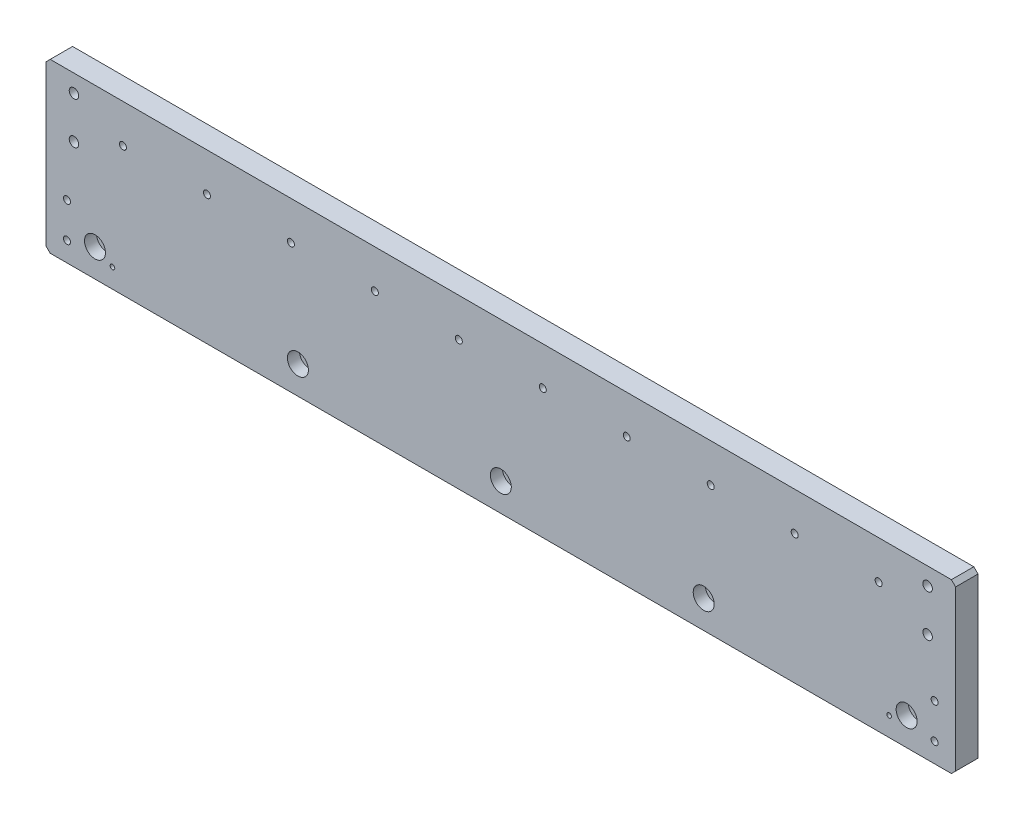
from build123d import *

# Parameters (mm, degrees)
SKETCH_1_W                     = 670
SKETCH_1_H                     = 140
EXTRUDE_1_DEPTH                = 16
HOLE_WIZARD_M8_1_D             = 6.8
HOLE_WIZARD_M6_1_D             = 5
HOLE_WIZARD_M8_1_2_D           = 9
HOLE_WIZARD_M8_1_2_CBORE_D     = 15
HOLE_WIZARD_M8_1_2_CBORE_DEPTH = 8.6
SKETCH_16_W                    = 670
SKETCH_16_H                    = 20
CUT_EXTRUDE_1_DEPTH            = 343.609106709
SKETCH_19_W                    = 10
SKETCH_19_H                    = 120
CUT_EXTRUDE_2_DEPTH            = 343.609106709
CHAMFER_1_SIZE                 = 3
HOLE_WIZARD_M6_2_D             = 5
HOLE_WIZARD_M4_1_D             = 3.3


with BuildPart() as part:
    # 草图1 → 凸台-拉伸1 (new body)
    with BuildSketch(Plane.XY):
        Rectangle(SKETCH_1_W, SKETCH_1_H)
    extrude(amount=EXTRUDE_1_DEPTH)

    # Hole Wizard M8 _1 (through all)
    with Locations(Plane.XY.offset(16)):
        with Locations((-305, 57.5), (-305, 27.5), (305, 27.5), (305, 57.5)):
            Hole(HOLE_WIZARD_M8_1_D / 2)

    # M6 螺纹孔1 (through all)
    with Locations(Plane.XY.offset(16)):
        with Locations((-270, 42.5), (-210, 42.5), (-150, 42.5), (-90, 42.5), (-30, 42.5), (30, 42.5), (90, 42.5), (150, 42.5), (210, 42.5), (270, 42.5)):
            Hole(HOLE_WIZARD_M6_1_D / 2)

    # Hole Wizard M8 _1 2 (through all)
    with Locations(Plane.XY.offset(16)):
        with Locations((290, -30), (145, -30), (0, -30), (-145, -30), (-290, -30), (-435, -30)):
            CounterBoreHole(HOLE_WIZARD_M8_1_2_D / 2, HOLE_WIZARD_M8_1_2_CBORE_D / 2, HOLE_WIZARD_M8_1_2_CBORE_DEPTH)

    # 草图16 → 切除-拉伸1 (cut, through all)
    with BuildSketch(Plane.XY.offset(16)):
        with Locations((0, -60)):
            Rectangle(SKETCH_16_W, SKETCH_16_H)
    extrude(amount=-CUT_EXTRUDE_1_DEPTH, mode=Mode.SUBTRACT)

    # 草图19 → 切除-拉伸2 (cut, through all)
    with BuildSketch(Plane.XY.offset(16)):
        with Locations((-330, 10)):
            Rectangle(SKETCH_19_W, SKETCH_19_H)
    cut_extrude_2 = extrude(amount=-CUT_EXTRUDE_2_DEPTH, mode=Mode.SUBTRACT)

    # 镜向1: 切除-拉伸2 across plane
    add(cut_extrude_2.mirror(Plane(origin=(0, 0, 0), x_dir=(0, 0, 1), z_dir=(1, 0, 0))), mode=Mode.SUBTRACT)

    # 倒角1
    chamfer_1_edges = [part.edges().sort_by_distance(p)[0] for p in [
        (-325, 70, 8),
        (-325, -50, 8),
        (325, -50, 8),
        (325, 70, 8),
    ]]
    chamfer(chamfer_1_edges, length=CHAMFER_1_SIZE)

    # M6 螺纹孔2 (through all)
    with Locations(Plane.XY.offset(16)):
        with Locations((-310, -11), (-310, -36), (310, -11), (310, -36)):
            Hole(HOLE_WIZARD_M6_2_D / 2)

    # M4 螺纹孔1 (through all)
    with Locations(Plane.XY.offset(16)):
        with Locations((277.5, -36.25), (-277.5, -36.25)):
            Hole(HOLE_WIZARD_M4_1_D / 2)


solid = part.part
